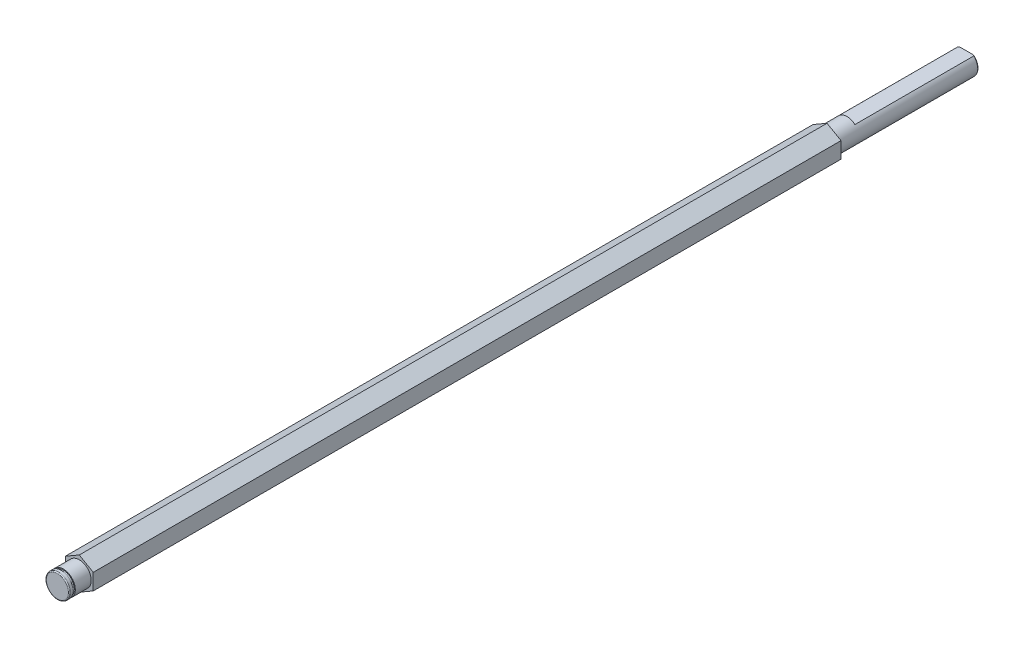
from build123d import *

# Parameters (mm, degrees)
EXTRUDE_1_DEPTH     = 375
SKETCH_2_R          = 6
EXTRUDE_2_DEPTH     = 70
EXTRUDE_START       = 11
SKETCH_3_R          = 6
EXTRUDE_3_DEPTH     = 11
FILLET_1_R          = 0.5
SKETCH_6_W          = 1
SKETCH_6_H          = 1.1
FILLET_2_R          = 0.5
SKETCH_7_W          = 10
SKETCH_7_H          = 2
CUT_EXTRUDE_1_DEPTH = 60


with BuildPart() as part:
    # 草图1 → 凸台-拉伸1 (new body)
    with BuildSketch(Plane.XY):
        Polygon((7, -4.041451884), (7, 4.041451884), (0, 8.082903769), (-7, 4.041451884), (-7, -4.041451884), (0, -8.082903769), align=None)
    extrude(amount=EXTRUDE_1_DEPTH)

    # 草图2 → 凸台-拉伸2 (add)
    with BuildSketch(Plane(origin=(0, 0, 0), x_dir=(-1, 0, 0), z_dir=(0, 0, -1))):
        with Locations(Location((0, 0, 0), (0, 0, 180))):
            Circle(SKETCH_2_R)
    extrude(amount=EXTRUDE_2_DEPTH)

    # 草图3 → 凸台-拉伸3 (add)
    with BuildSketch(Plane.XY.offset(375).offset(EXTRUDE_START)):
        Circle(SKETCH_3_R)
    extrude(amount=-EXTRUDE_3_DEPTH)

    # 圆角1
    fillet_1_edges = [part.edges().sort_by_distance(p)[0] for p in [
        (-6, 0, -70),
    ]]
    fillet(fillet_1_edges, radius=FILLET_1_R)

    # 草图6 → 切除-旋转2 (revolve, cut)
    with BuildSketch(Plane(origin=(0, 0, 0), x_dir=(1, 0, 0), z_dir=(0, 1, 0)), mode=Mode.PRIVATE) as cut_revolve_2_sk:
        with Locations((6, -383.55)):
            Rectangle(SKETCH_6_W, SKETCH_6_H)
    revolve(cut_revolve_2_sk.sketch.rotate(Axis((0, 0, 418.9281299), (0, 0, -1)), 180), axis=Axis((0, 0, 418.9281299), (0, 0, -1)), mode=Mode.SUBTRACT)

    # 圆角2
    fillet_2_edges = [part.edges().sort_by_distance(p)[0] for p in [
        (-6, 0, 386),
    ]]
    fillet(fillet_2_edges, radius=FILLET_2_R)

    # 草图7 → 切除-拉伸1 (cut)
    with BuildSketch(Plane(origin=(0, 0, -70), x_dir=(-1, 0, 0), z_dir=(0, 0, -1))):
        with Locations((0, 5.5)):
            Rectangle(SKETCH_7_W, SKETCH_7_H)
    extrude(amount=-CUT_EXTRUDE_1_DEPTH, mode=Mode.SUBTRACT)


solid = part.part
